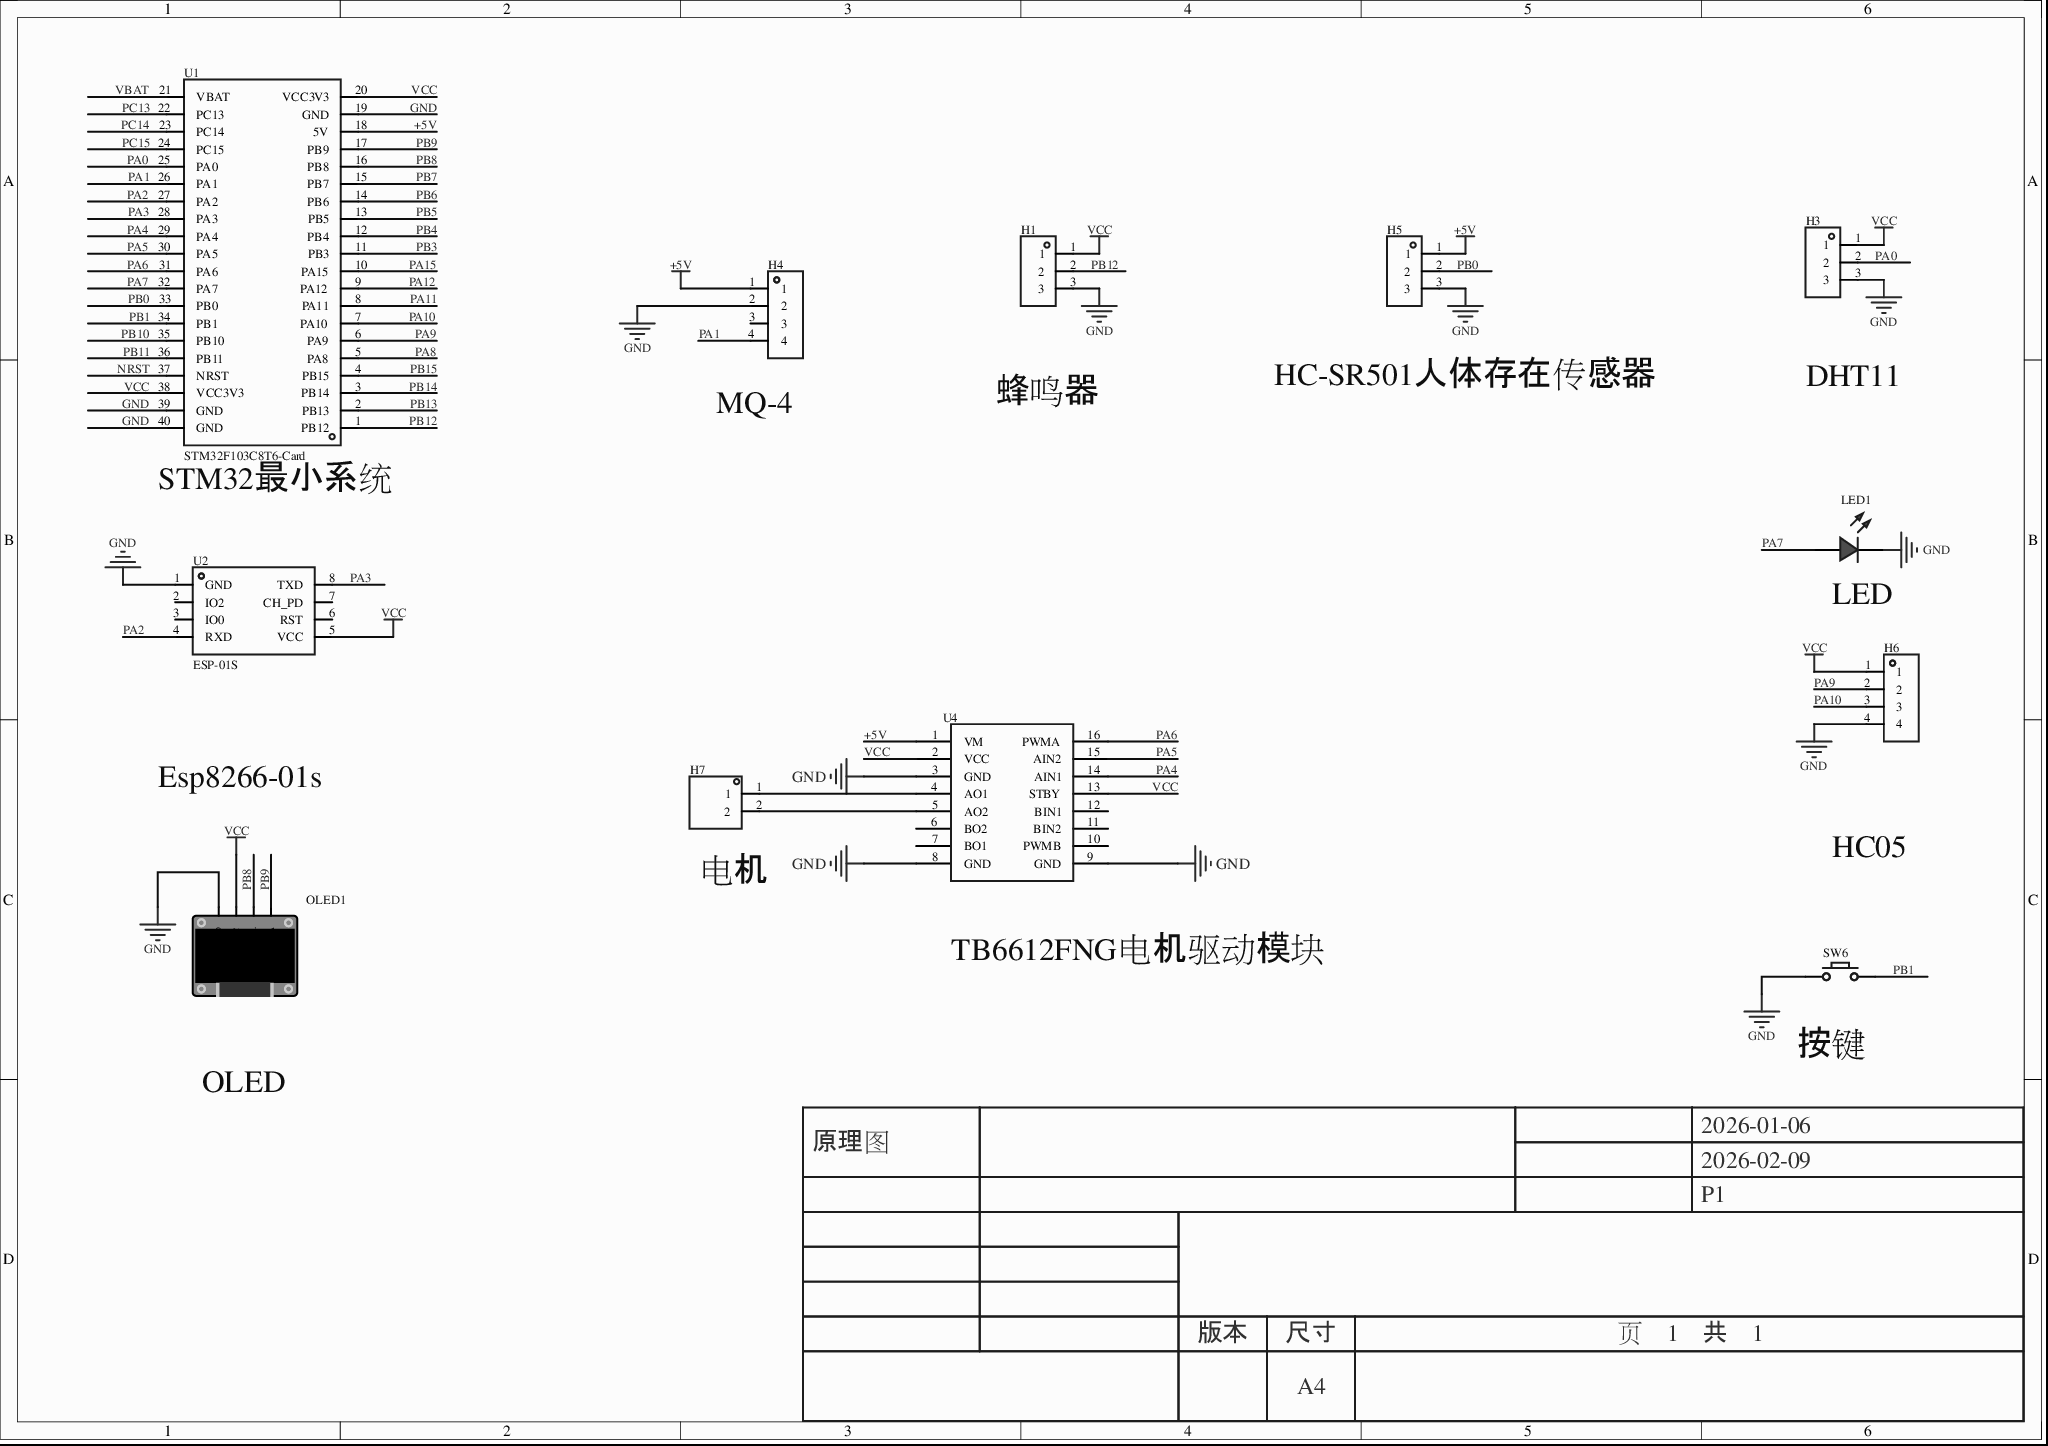
[diagram p0: MISC50942-3.schdoc]
# Altium project MISC50942-2.PrjPcb
1 sheet, 12 parts. Net scope: global (net labels, ports and power ports of the same name join across sheets).
Board file: MISC50942.pcbdoc

## Sheet MISC50942-3.schdoc
size 297 x 209 mm; Version: V1.0; @Project Name: MISC50942; @Page Count: 1; @Update Date: 2026-04-13; @Create Date: 2026-04-13; @Schematic Name: MISC50942; @Page No: 1; @Create Time: 23:22:16; @Update Time: 17:32:40; @Board Name: MISC50942

### Parts
H1  (no value)  [HDR-TH_3P-P2.54-V-F]
H3  (no value)  [HDR-TH_3P-P2.54-V-F]
H4  (no value)  [HDR-TH_4P-P2.54-V-F]
H5  (no value)  [HDR-TH_3P-P2.54-V-F]
H6  (no value)  [HDR-TH_4P-P2.54-V-F]
H7  (no value)  [HDR-TH_2P-P2.54-V-M-1]
LED1  (no value)  [LED_TH-3mm]
OLED1  (no value)  [0.96OLED_4P]
SW6  (no value)  [Key_TH_3.5x6x4.3]
U1  STM32F103C8T6-Card  [CONN-TH_L53.3-W22.9_STM32F103C8T6-CARD]
U2  ESP-01S  [WIFIM-TH_ESP-01S]
U4  (no value)  [tb6612]

### Nets
+5V: H4.1 H5.1 U1.18(5V) U4.1(VM)
GND: H1.3 H3.3 H4.2 H5.3 H6.4 LED1.2(A) OLED1.1(GND) SW6.A U1.19(GND) U1.39(GND) U1.40(GND) U2.1(GND) U4.3(GND) U4.8(GND) U4.9(GND)
VCC: H1.1 H3.1 H6.1 OLED1.2(VCC) U1.20(VCC3V3) U1.38(VCC3V3) U2.5(VCC) U4.2(VCC) U4.13(STBY)
NRST: U1.37(NRST)
PA0: H3.2 U1.25(PA0)
PA1: H4.4 U1.26(PA1)
PA2: U1.27(PA2) U2.4(RXD)
PA3: U1.28(PA3) U2.8(TXD)
PA4: U1.29(PA4) U4.14(AIN1)
PA5: U1.30(PA5) U4.15(AIN2)
PA6: U1.31(PA6) U4.16(PWMA)
PA7: LED1.1(C) U1.32(PA7)
PA8: U1.5(PA8)
PA9: H6.2 U1.6(PA9)
PA10: H6.3 U1.7(PA10)
PA11: U1.8(PA11)
PA12: U1.9(PA12)
PA15: U1.10(PA15)
PB0: H5.2 U1.33(PB0)
PB1: SW6.B U1.34(PB1)
PB3: U1.11(PB3)
PB4: U1.12(PB4)
PB5: U1.13(PB5)
PB6: U1.14(PB6)
PB7: U1.15(PB7)
PB8: OLED1.3(SCL) U1.16(PB8)
PB9: OLED1.4(SDA) U1.17(PB9)
PB10: U1.35(PB10)
PB11: U1.36(PB11)
PB12: H1.2 U1.1(PB12)
PB13: U1.2(PB13)
PB14: U1.3(PB14)
PB15: U1.4(PB15)
PC13: U1.22(PC13)
PC14: U1.23(PC14)
PC15: U1.24(PC15)
VBAT: U1.21(VBAT)
NetH7_1: H7.1 U4.4(AO1)
NetH7_2: H7.2 U4.5(AO2)

Not connected (* = marked no-connect by the designer): H4 3; U2 2(IO2)* 3(IO0)* 6(RST)* 7(CH_PD)*; U4 6(BO2) 7(BO1) 10(PWMB) 11(BIN2) 12(BIN1)

### Notes on the sheet
- (near H4) MQ-4
- 蜂鸣器
- HC-SR501人体存在传感器
- DHT11
- (near U1) STM32最小系统
- (near LED1) LED
- Esp8266-01s
- HC05
- (near H7) 电机
- TB6612FNG电机驱动模块
- OLED
- (near SW6) 按键
- 2026-01-06
- 原理图
- 2026-02-09
- P1
- 版本
- 尺寸
- A4
- 页    1    共    1

### Library data of the parts
H1 H3 H5 = HDR-F_2.54_1x3P: Symbol: PM254V-11-03-H85; 3D Model: f3b3cc5aae9641bf9e56fc160cef875b; 3D Model Transform: 299.9994,100,0,0,0,0,0,0,-118.11; ConvertToPcb: yes; ModelName: HDR2.54-F-LI-1X3P; Device: HDR-F_2.54_1x3P; Supplier Part: C541850; Supplier Footprint: 插件; FootprintName: HDR-TH_3P-P2.54-V-F; AddInBom: yes
H4 = HDR-F_2.54_1x4P: Symbol: 2.54-1*4P母; ConvertToPcb: yes; ModelId: d187812051054f85879fcaa51a310d8e0819f05c4eef4c71ace90d822a990e87; ModelTransform: 419.6842,98.464,0,0,0,0,0,0,-118.11; Device: HDR-F_2.54_1x4P; FootprintName: HDR-TH_4P-P2.54-V-F; AddInBom: yes; SupplierPart: C2718488; Supplier Footprint: 插件; ModelName: HDR-TH_4P-P2.54-V-F
H6 = HDR-F_2.54_1x4P: Symbol: 2.54-1*4P母; 3D Model: d187812051054f85879fcaa51a310d8e0819f05c4eef4c71ace90d822a990e87; 3D Model Transform: 419.6842,98.464,0,0,0,0,0,0,-118.11; ConvertToPcb: yes; Device: HDR-F_2.54_1x4P; Supplier Part: C2718488; Supplier Footprint: 插件; FootprintName: HDR-TH_4P-P2.54-V-F; AddInBom: yes; ModelName: HDR-TH_4P-P2.54-V-F
H7 = HDR-M_2.54_1x2P: Symbol: 210S-1*2P L=11.6MMGold-plated black; ConvertToPcb: yes; ModelId: 79b2e9f2d70a4d68a1b7098f27c6d4c50819f05c4eef4c71ace90d822a990e87; ModelName: HDR-M-2.54_1x2; ModelTransform: 200,100,0,0,0,0,0,0,-118.11; Device: HDR-M_2.54_1x2P; AddInBom: yes; SupplierPart: C124375; Supplier Footprint: 插件; FootprintName: HDR-TH_2P-P2.54-V-M-1
LED1 = LED_TH-R_3mm: ConvertToPcb: yes; ModelId: a497c992633541038a38947cdc58012f0819f05c4eef4c71ace90d822a990e87; ModelName: LED-TH-3mm_R; ModelTransform: 141.274,153.327,0,0,0,0,-5.984,0,-137.795; Symbol: LED_TH-R; Device: LED_TH-R_3mm; AddInBom: yes; FootprintName: LED_TH-3mm; Supplier Footprint: 插件
OLED1 = 0.96OLED模块_4P: ConvertToPcb: yes; ModelId: 79c000fdb68d45a296c2e9bedf4f9055; ModelTransform: 1393.69792,1318.895,0,0,0,0,0,-560.079,-137.795; Symbol: 0.96OLED模块_4P; Device: 0.96OLED模块_4P; AddInBom: yes; FootprintName: 0.96OLED_4P; Supplier Footprint: 插件; ModelName: 0.96OLED_4P
SW6 = Key_TH_3.5x6x4.3: ConvertToPcb: yes; ModelId: c3523f9014d949d7ba5445190a3178990819f05c4eef4c71ace90d822a990e87; ModelName: SW-TH_L6.0-W3.5-H5.0-P6.5; ModelTransform: 308.49,137.8,335.08,0,0,0,0,0,-129.92; Symbol: Key_TH_3.5x6x4.3; Device: Key_TH_3.5x6x4.3; AddInBom: yes; Supplier Footprint: 插件; FootprintName: Key_TH_3.5x6x4.3
U1 = STM32F103C8T6-Card: AddInBom: yes; Device: STM32F103C8T6-Card; Symbol: STM32F103C8T6-CARD; FootprintName: CONN-TH_L53.3-W22.9_STM32F103C8T6-CARD; LCSC Part Name: STM32F103C8T6-Card; SupplierPart: C9900077949; ManufacturerPart: STM32F103C8T6-Card; Supplier Footprint: 插件; Supplier: LCSC; ConvertToPcb: yes
U2 = ESP-01S_C111009: 3D Model: eb7175da78ae48b3b1568cfe3027405f0819f05c4eef4c71ace90d822a990e87; 3D Model Transform: 582.676,976.37608,0,0,0,0,0,388.346,-118.11; AddInBom: yes; Symbol: ESP-01S; Device: ESP-01S_C111009; LCSC Part Name: ESP-01S; Supplier Part: C111009; Manufacturer Part: ESP-01S; Supplier Footprint: -; JLCPCB Part Class: Extended Part; Supplier: LCSC; ConvertToPcb: yes; FootprintName: WIFIM-TH_ESP-01S; ModelName: WIFIM-TH_ESP-01S
U4 = tb6612: AddInBom: yes; Symbol: tb6612; Device: tb6612; JLCPCB Part Class: 扩展库; ConvertToPcb: yes; FootprintName: tb6612